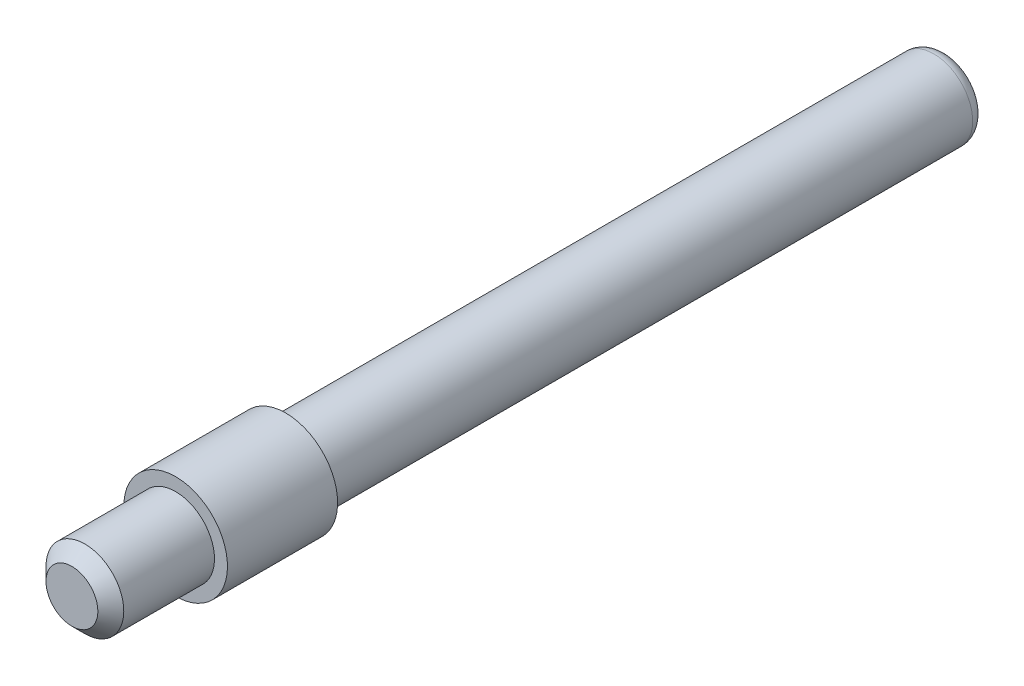
SolidWorks part; units mm, degrees
material "米黄色赛刚"
ref_plane "前视基准面" through (0, 0, 0) normal (0, 0, 1) x (1, 0, 0)
ref_plane "上视基准面" through (0, 0, 0) normal (0, 1, 0) x (1, 0, 0)
ref_plane "右视基准面" through (0, 0, 0) normal (1, 0, 0) x (0, 0, -1)
sketch "草图1" plane through (0, 0, 0) normal (1, 0, 0) x (0, 0, -1)
  line L0 (0, 0) -> (0, 3)
  line L1 (0, 3) -> (8, 3)
  line L2 (8, 3) -> (8, 4)
  line L3 (8, 4) -> (16.5, 4)
  line L4 (16.5, 4) -> (16.5, 3)
  line L5 (16.5, 3) -> (67.5, 3)
  line L6 (67.5, 3) -> (67.5, 0)
  line L7 (67.5, 0) -> (0, 0)
  dimension "D1" = 3
  dimension "D2" = 4
  dimension "D3" = 8
  dimension "D4" = 8.5
  dimension "D5" = 51
revolve "旋转1" add sketch "草图1" angle 360 about L7
fillet "圆角1" radius 1 1 edges at (0, 3, -67.5)
chamfer "倒角1" distance 1 angle 45 1 edges at (0, 3, 0)
